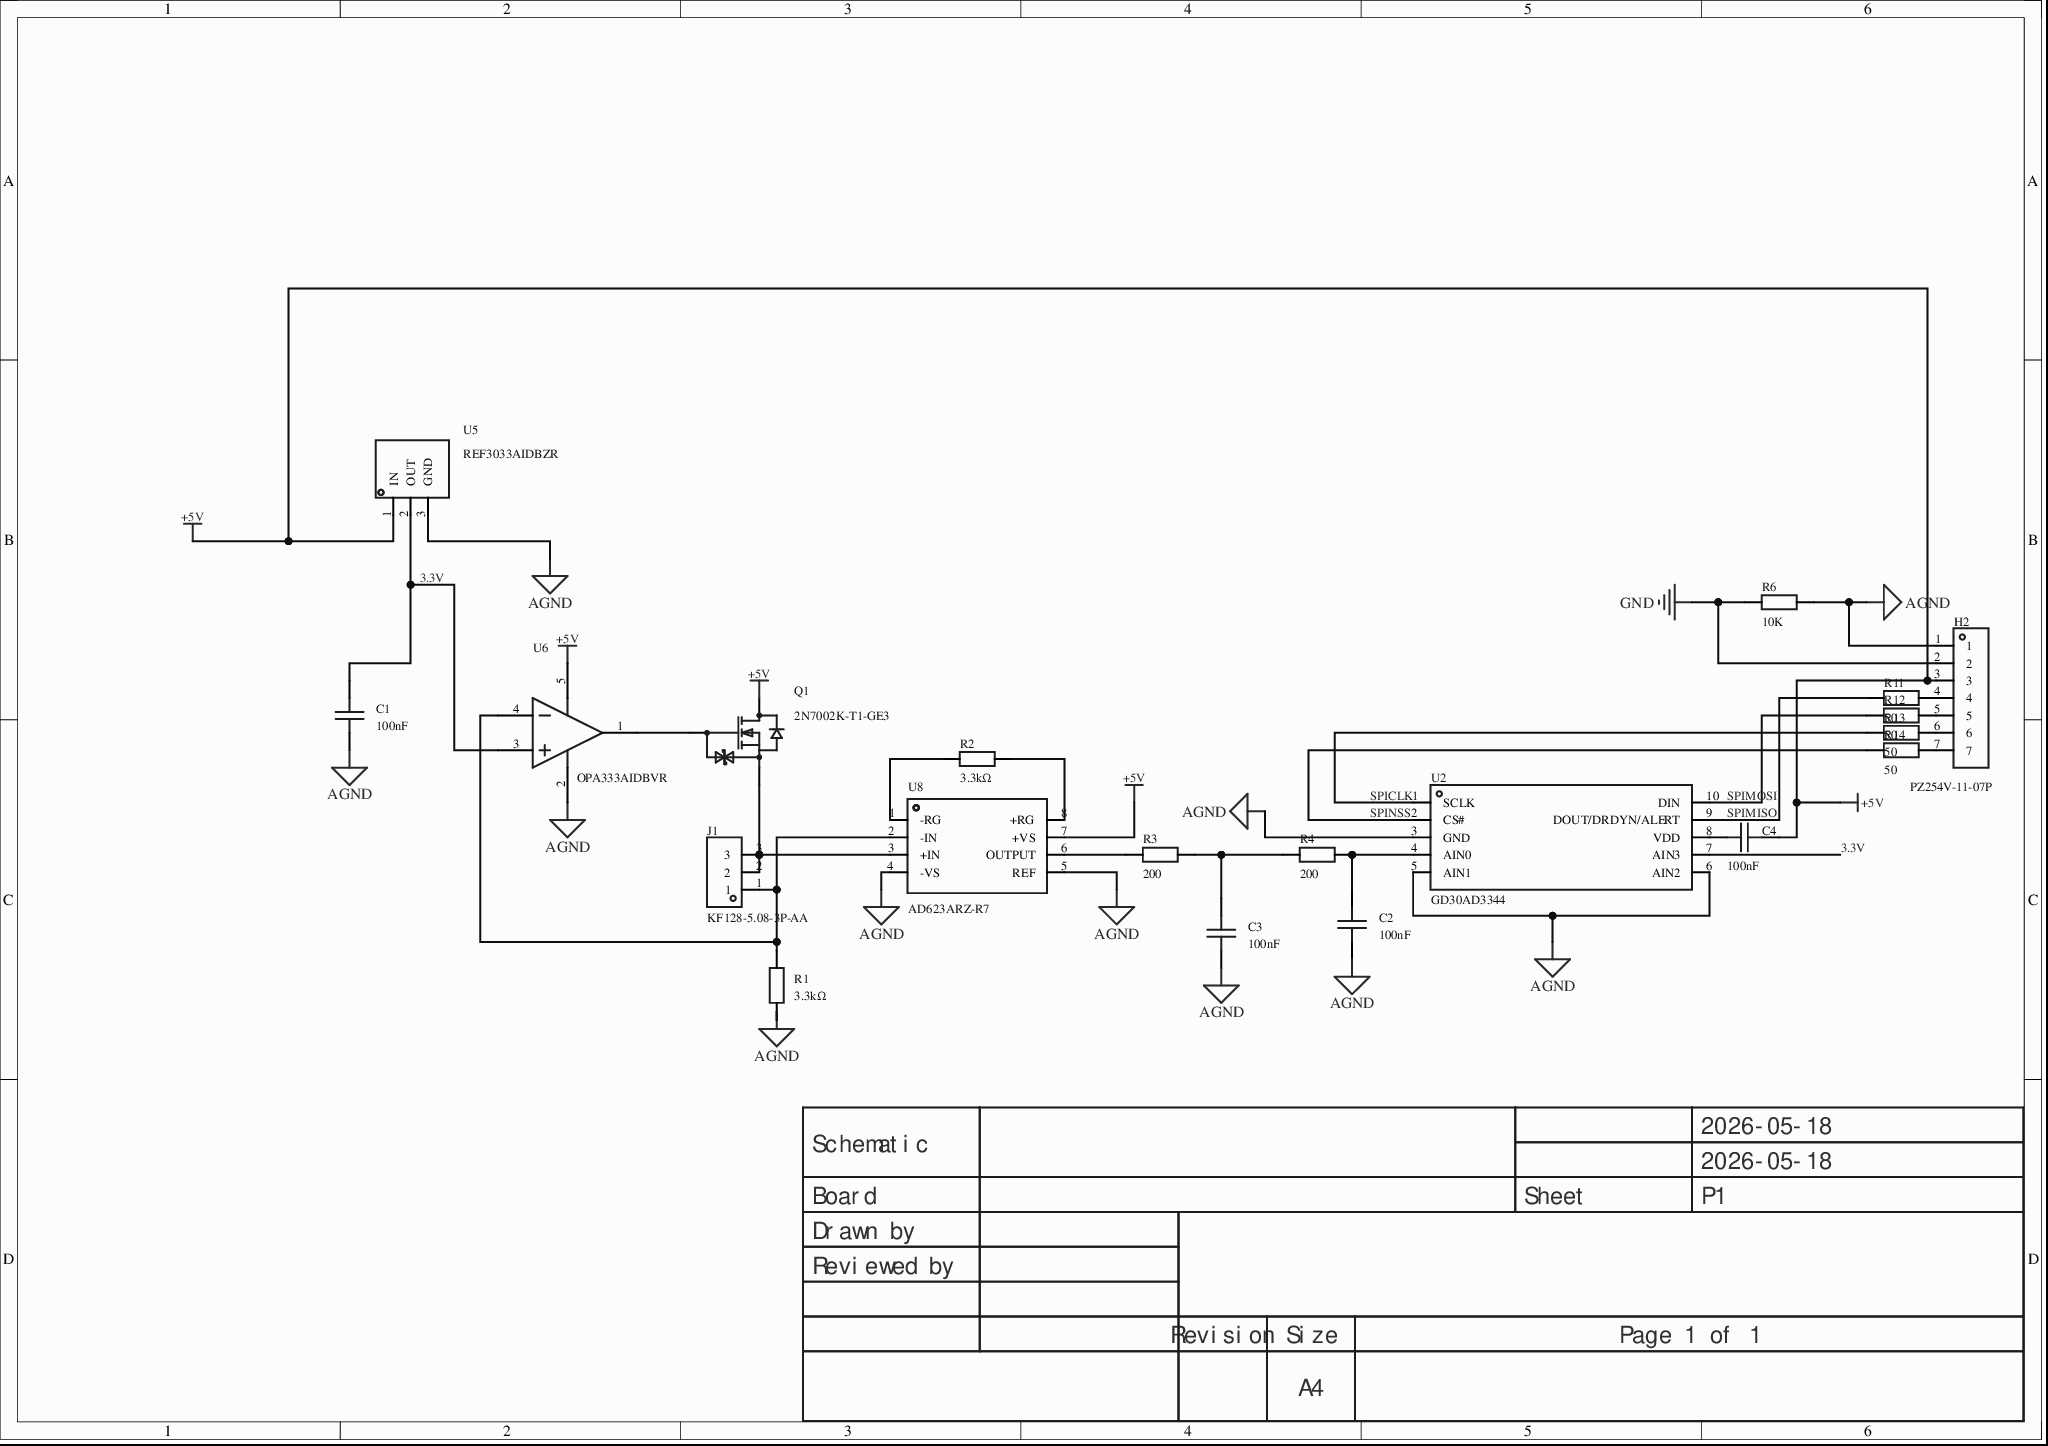
[diagram p0: MISC51892-3.schdoc]
# Altium project MISC51892-2.PrjPcb
1 sheet, 20 parts. Net scope: global (net labels, ports and power ports of the same name join across sheets).
Board file: MISC51892.pcbdoc

## Sheet MISC51892-3.schdoc
size 297 x 209 mm; Version: V1.0; @Project Name: MISC51892; @Page Count: 1; @Update Date: 2026-05-18; @Create Date: 2026-05-18; @Schematic Name: MISC51892; @Page No: 1; @Board Name: MISC51892; @Create Time: 13:05:29; @Update Time: 09:04:01; Size: A4

### Parts
C1  100nF  [C0805]
C2  100nF  [C0805]
C3  100nF  [C0805]
C4  100nF  [C0805]
H2  PZ254V-11-07P  [HDR-TH_7P-P2.54-V-M]
J1  KF128-5.08-3P-AA  [CONN-TH_3P-P5.08_KF128-5.08-3P]
Q1  2N7002K-T1-GE3  [SOT-23-3_L2.9-W1.6-P1.90-LS2.8-BR]
R1  3.3kΩ  [Res_1/4W]
R2  3.3kΩ  [Res_1/4W]
R3  200  [Res_1/4W]
R4  200  [Res_1/4W]
R6  10K  [Res_1/4W]
R11  50  [R0805]
R12  50  [R0805]
R13  50  [R0805]
R14  50  [R0805]
U2  GD30AD3344  [MSOP-10_L3.0-W3.0-P0.50-LS5.0-BL]
U5  REF3033AIDBZR  [SOT-23-3_L3.0-W1.7-P0.95-LS2.9-BR]
U6  OPA333AIDBVR  [SOT-23-5_L3.0-W1.7-P0.95-LS2.8-BR]
U8  AD623ARZ-R7  [SOIC-8_L5.0-W4.0-P1.27-LS6.0-BL]

### Nets
+5V: C4.2 H2.3 Q1.3(D) U5.1(IN) U6.5(V+) U8.7(+VS)
AGND: C1.1 C2.1 C3.1 H2.1 R1.1 R6.2 U2.3(GND) U2.5(AIN1) U2.6(AIN2) U5.3(GND) U6.2(V-) U8.4(-VS) U8.5(REF)
GND: H2.2 R6.1
3.3V: C1.2 U2.7(AIN3) U5.2(OUT) U6.3(IN+)
SPICLK: R13.1 U2.1(SCLK)
SPIMISO: R11.1 U2.9(DOUT/DRDYN/ALERT)
SPIMOSI: R12.1 U2.10(DIN)
SPINSS: R14.1 U2.2(CS#)
NetC2_2: C2.2 R4.2 U2.4(AIN0)
NetC3_2: C3.2 R3.2 R4.1
NetC4_1: C4.1 U2.8(VDD)
NetH2_4: H2.4 R11.2
NetH2_5: H2.5 R12.2
NetH2_6: H2.6 R13.2
NetH2_7: H2.7 R14.2
NetJ1_1: J1.1 R1.2 U6.4(IN-) U8.2(-IN)
NetJ1_2: J1.2 J1.3 Q1.2(S) U8.3(+IN)
NetQ1_1: Q1.1(G) U6.1(OUT)
NetR2_1: R2.1 U8.1(-RG)
NetR2_2: R2.2 U8.8(+RG)
NetR3_1: R3.1 U8.6(OUTPUT)

### Notes on the sheet
- 2026-05-18
- Schematic
- Board
- Sheet
- P1
- Drawn by
- Reviewed by
- Revision
- Size
- A4
- Page 1 of 1

### Library data of the parts
C1-C4 = CAP_0805: ConvertToPcb: yes; SymbolName: Capacitance; ModelId: 1ba041120af144c991958decab20d241; ModelName: C0805_L2.0-W1.3-H1.3; ModelTransform: 78.74,51.181,0,0,0,0,0,0.0005,0; Device: CAP_0805; AddInBom: yes; Supplier Footprint: 0805; FootprintName: C0805; Value: 100nF
H2 = PZ254V-11-07P: 插针结构:1x7P;间距:2.54mm;行距:-;圆针/方针:方针;安装方式:直插;排数:单排;总PIN位数:7P;额定电流:3A;额定电压:250V;配合针长度:6mm;塑高:2.5mm;端接针长度:3mm;触头材质:黄铜;触头镀层:-;工作温度:-40℃~+105℃;颜色:黑色;; Manufacturer: XFCN(兴飞); AddInBom: yes; ModelId: 3f496cdc752348c6a5e9157bbaceaf96; ModelName: HDR-TH_7P-P2.54-M-LI-1X7P; ModelTransform: 690.1561,98.425,0,0,0,0,0,0,-118.11; Pin Structure: 1x7P; Pitch: 2.54mm; Circluar Pins/Square Pins: Square pin; Current Rating: 3A; Voltage Rating (Max): 250V; Symbol: PZ254V-11-07P; Device: PZ254V-11-07P; LCSC Part Name: 1x7P 间距:2.54mm 方针 直插; SupplierPart: C492406; ManufacturerPart: PZ254V-11-07P; Supplier Footprint: 插件,P=2.54mm; JLCPCB Part Class: Extended library; Datasheet: https://item.szlcsc.com/datasheet/PZ254V-11-07P/502962.html; Supplier: LCSC; ConvertToPcb: yes; FootprintName: HDR-TH_7P-P2.54-V-M; Row Spacing: -; Mounting Type: Through-hole; Number of Rows: Single row; Number of Pins: 7P; Length of Mating Pin: 6mm; Insulation Height: 2.5mm; Length of End Connection Pin: 3mm; Contact Material: Brass; Contact Plating: -; Operating Temperature: -40℃~+105℃; Color: Black
J1 = KF128-5.08-3P-AA: 结构:1x3P;间距:5.08mm;颜色:绿色;安装方式:直插;排数:1;每排PIN数:3;额定电流:24A;额定电压:250V;线规 - AWG:12~22;线规 - 平方毫米:2.5;工作温度:-40℃~+105℃;; Manufacturer: KEFA(科发); AddInBom: yes; ModelId: a265b55f168f4366b002141bfacab5d1; ModelTransform: 623.62474,421.259,0,180,0,0,11.811,1.968,-137.795; Number of Positions or Pins: 1x3P; Pitch: 5.08mm; Number of PINs Per Row: 3; Current Rating: 24A; Voltage Rating (Max): 250V; Wire Gauge - AWG: 12~22; Wire Gauge - mm2: 2.5; Symbol: KF128-5.08-3P; Device: KF128-5.08-3P-AA; LCSC Part Name: 1x3P 5.08mm 直插 排数:1 每排P数:3; SupplierPart: C474953; ManufacturerPart: KF128-5.08-3P-AA; Supplier Footprint: 插件,P=5.08mm; JLCPCB Part Class: Extended library; Datasheet: https://item.szlcsc.com/datasheet/KF128-5.08-3P-AA/481571.html; Supplier: LCSC; ConvertToPcb: yes; FootprintName: CONN-TH_3P-P5.08_KF128-5.08-3P; ModelName: CONN-TH_3P-P5.08_KF128-5.08-3P; Color: Green; Mounting Type: Through-hole; Number of Pins: 3P; Number of Rows: 1; Operating Temperature: -40℃~+105℃
Q1 = 2N7002K-T1-GE3: 数量:1个N沟道;漏源电压(Vdss):60V;连续漏极电流(Id):300mA;导通电阻(RDS(on)):2Ω@10V,500mA;耗散功率(Pd):350mW;阈值电压(Vgs(th)):2.5V;; Manufacturer: VISHAY(威世); AddInBom: yes; ModelId: 89cb27a44ab2466697082bb9fd73a7d0; ModelName: SOT-23-3L_L2.9-W1.6-H1.1-LS2.8-P0.95; ModelTransform: 114.173,110.236,0,90,0,0,0,0,0; Number: 1 N-channel; Drain to Source Voltage: 60V; Current - Continuous Drain(Id): 300mA; Pd - Power Dissipation: 350mW; Gate Threshold Voltage (Vgs(th)): 2.5V; Gate Charge(Qg): 600pC@10V; Reverse Transfer Capacitance (Crss@Vds): 2.5pF@10V; Symbol: 2N7002K-T1-GE3; Device: 2N7002K-T1-GE3; LCSC Part Name: 1个N沟道 耐压:60V 电流:300mA; SupplierPart: C81445; ManufacturerPart: 2N7002K-T1-GE3; Supplier Footprint: SOT-23; JLCPCB Part Class: Extended library; Datasheet: https://item.szlcsc.com/datasheet/2N7002K-T1-GE3/82596.html; Supplier: LCSC; ConvertToPcb: yes; FootprintName: SOT-23-3_L2.9-W1.6-P1.90-LS2.8-BR; RDS(on): 2Ω@10V,500mA; Input Capacitance(Ciss): -; Operating Temperature: -55℃~+150℃
R1-R4 R6 = Res_AXIAL-1/4W: AddInBom: yes; SymbolName: Resistor; ModelId: 463263665006444ab7a47bd11b0cf956; ModelName: RES-TH_BD2.4-L6.3-P10.30-D0.6; ModelTransform: 427.165,94.32816,0,0,0,0,0,0,-196.85; Device: Res_AXIAL-1/4W; Supplier Footprint: 轴向引线; ConvertToPcb: yes; FootprintName: Res_1/4W
  R1 R2: Value: 3.3kΩ
  R3 R4: Value: 200
  R6: Value: 10K
R11-R14 = Res_0805: ConvertToPcb: yes; SymbolName: Resistor; ModelId: 37a81e68749a4138bd2dfa6897b24b85; ModelName: R0805_L2.0-W1.3-H0.6; ModelTransform: 78.74,51.181,0,0,0,0,0,-0.0005,0; Value: 50; Device: Res_0805; AddInBom: yes; Supplier Footprint: 0805; FootprintName: R0805
U2 = GD30AD3344: AddInBom: yes; ModelId: b42a31f9e1fa4643bc7ea573b9bba7ed; ModelName: MSOP-10_L3.0-W3.0-H1.1-LS5.0-P0.50; ModelTransform: 118.11,196.85,0,0,0,0,0,0,0; Symbol: GD30AD3344; Device: GD30AD3344; LCSC Part Name: GD30AD3344; SupplierPart: C9900209500; ManufacturerPart: GD30AD3344; Supplier Footprint: MSOP-10; Supplier: LCSC; ConvertToPcb: yes; FootprintName: MSOP-10_L3.0-W3.0-P0.50-LS5.0-BL
U5 = REF3033AIDBZR: 输出类型:固定;工作电压:3.35V~5.5V;输出电压:3.3V;输出电流:25mA;精度:±0.2%;; Manufacturer: TI(德州仪器); AddInBom: yes; ModelId: 89cb27a44ab2466697082bb9fd73a7d0; ModelName: SOT-23-3L_L2.9-W1.6-H1.1-LS2.8-P0.95; ModelTransform: 114.173,110.236,0,90,0,0,0,0,0; Output Type: Fixed; Output Voltage: 3.3V; Output Current: 25mA; Tolerance: ±0.2%; Temperature Coefficient: 75ppm/℃; Reference Type: Series; Quiescent Current: 50uA; Noise - 1/10Hz to 10Hz: 36uVp-p; Noise - 10Hz to 10kHz: 105uVrms; Symbol: REF3033AIDBZR; Device: REF3033AIDBZR; LCSC Part Name: 3.35V~5.5V 串联 50uA 75ppm/℃; SupplierPart: C36658; ManufacturerPart: REF3033AIDBZR; Supplier Footprint: SOT-23; JLCPCB Part Class: Extended library; Supplier: LCSC; ConvertToPcb: yes; FootprintName: SOT-23-3_L3.0-W1.7-P0.95-LS2.9-BR; Voltage - Supply: 3.35V~5.5V; Minimum Cathode Current for Regulation: -; Operating Temperature: -40℃~+125℃@(Ta)
U6 = OPA333AIDBVR: 放大器数:单路;增益带宽积(GBP):350kHz;输入偏置电流(Ib):70pA;输入失调电压(Vos):2uV;压摆率(SR):0.16V/us;轨到轨:轨到轨输入,轨到轨输出;; Manufacturer: TI(德州仪器); AddInBom: yes; ModelId: 0a2a1b8f50944f73965918ad6e5fe167; ModelName: SOT-23-5_L2.9-W1.6-H1.1-LS2.8-P0.95; ModelTransform: 114.173,109.636,0,180,0,0,0,0,0; Number of Channels: Single channel; Gain Bandwidth Product: 350kHz; Ib - Input Bias Current: 70pA; Vos - Input Offset Voltage: 2uV; Common Mode Rejection Ratio(CMRR): 130dB; Output Current: 5mA; Rail to Rail: Rail-to-rail input and output; Input Offset Voltage Drift(Vos TC): 50nV/℃; Quiescent Current(Iq): 17uA; Single Supply: 1.8V~5.5V; Dual Supply: 900mV~2.75V; -2.75V~-900mV; Maximum Power Supply Range (Vdd-Vss): 5.5V; Input Offset Current(Ios): 400pA; Symbol: OPA333AIDBVR; Device: OPA333AIDBVR; LCSC Part Name: OPAx333 1.8V微功耗CMOS运算放大器零漂移系列; SupplierPart: C30878; ManufacturerPart: OPA333AIDBVR; Supplier Footprint: SOT-23-5; JLCPCB Part Class: Extended library; Supplier: LCSC; ConvertToPcb: yes; FootprintName: SOT-23-5_L3.0-W1.7-P0.95-LS2.8-BR; Slew Rate: 0.16V/us; Operating Temperature: -40℃~+125℃
U8 = AD623ARZ-R7: 放大器数:单路;共模抑制比(CMRR):80dB;输入偏置电流(Ib):25nA;输入失调电压(Vos):200uV;增益带宽积(GBP):-;压摆率(SR):0.3V/us;轨到轨:轨到轨输出;; Manufacturer: ADI(亚德诺); AddInBom: yes; ModelId: 7abc64c95a1a4a04a4ef38f9097c870b; ModelTransform: 192.913,236.22,0,0,0,0,0,0,0; Number of Channels: Single channel; Common Mode Rejection Ratio(CMRR): 80dB; Ib - Input Bias Current: 25nA; Vos - Input Offset Voltage: 200uV; Rail to Rail: Rail-to-rail output; Quiescent Current(Iq): 550uA; Symbol: AD623ARZ-R7; Device: AD623ARZ-R7; LCSC Part Name: 单电源、轨到轨、低成本仪表放大器; SupplierPart: C9676; ManufacturerPart: AD623ARZ-R7; Supplier Footprint: SOIC-8; JLCPCB Part Class: Extended library; Datasheet: https://item.szlcsc.com/datasheet/AD623ARZ-R7/10206.html; Supplier: LCSC; ConvertToPcb: yes; FootprintName: SOIC-8_L5.0-W4.0-P1.27-LS6.0-BL; ModelName: SOIC-8_L5.0-W4.0-P1.27-LS6.0-BL; Gain Bandwidth Product: -; Slew Rate: 0.3V/us; Output Type: -; Operating Temperature: -40℃~+85℃